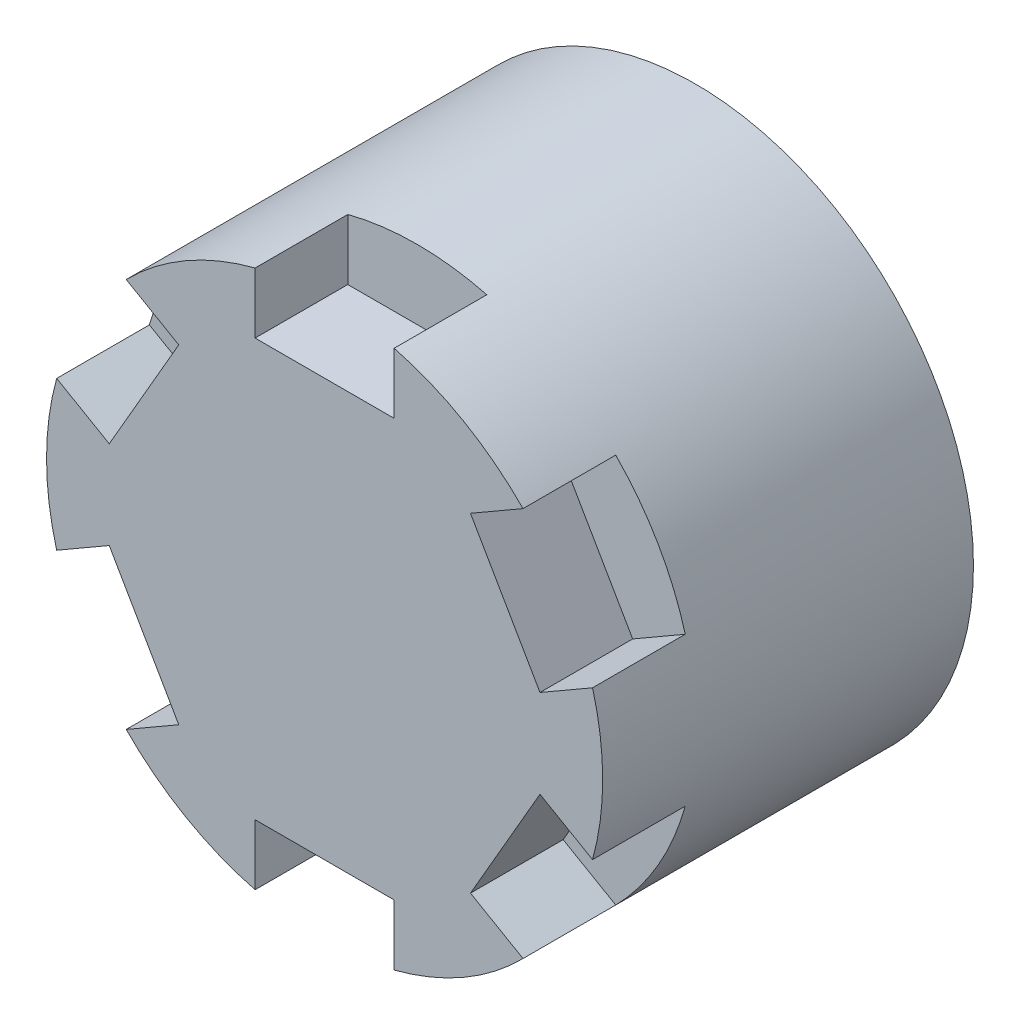
from build123d import *

# Parameters (mm, degrees)
SKETCH_2_R          = 60
EXTRUDE_1_DEPTH     = 80
SKETCH_1_R          = 37.5
CUT_EXTRUDE_1_DEPTH = 60
CUT_EXTRUDE_START   = -20
CUT_EXTRUDE_2_DEPTH = 20
SKETCH_4_W          = 20
SKETCH_4_H          = 11.668393693
CUT_EXTRUDE_3_DEPTH = 30


with BuildPart() as part:
    # 草图2 → 凸台-拉伸1 (new body)
    with BuildSketch(Plane.XY):
        Circle(SKETCH_2_R)
    extrude(amount=EXTRUDE_1_DEPTH)

    # 草图1 → 切除-拉伸1 (cut)
    with BuildSketch(Plane.XY):
        Circle(SKETCH_1_R)
    extrude(amount=CUT_EXTRUDE_1_DEPTH, mode=Mode.SUBTRACT)

    # 草图3 → 切除-拉伸2 (cut)
    with BuildSketch(Plane.XY.offset(80).offset(CUT_EXTRUDE_START)):
        with BuildLine():
            Line((57.811529494, 16.05699404), (46.47114317, 9.509618943))
            Line((46.47114317, 9.509618943), (31.47114317, 35.490381057))
            Line((31.47114317, 35.490381057), (42.811529494, 42.037756153))
            ThreePointArc((42.811529494, 42.037756153), (51.961524227, 30), (57.811529494, 16.05699404))
        make_face()
        with BuildLine():
            Line((-15, 58.094750193), (-15, 45))
            Line((-15, 45), (15, 45))
            Line((15, 45), (15, 58.094750193))
            ThreePointArc((15, 58.094750193), (0, 60), (-15, 58.094750193))
        make_face()
        with BuildLine():
            Line((42.811529494, -42.037756153), (31.47114317, -35.490381057))
            Line((31.47114317, -35.490381057), (46.47114317, -9.509618943))
            Line((46.47114317, -9.509618943), (57.811529494, -16.05699404))
            ThreePointArc((57.811529494, -16.05699404), (51.961524227, -30), (42.811529494, -42.037756153))
        make_face()
        with BuildLine():
            Line((-15, -58.094750193), (-15, -45))
            Line((-15, -45), (15, -45))
            Line((15, -45), (15, -58.094750193))
            ThreePointArc((15, -58.094750193), (0, -60), (-15, -58.094750193))
        make_face()
        with BuildLine():
            Line((-57.811529494, -16.05699404), (-46.47114317, -9.509618943))
            Line((-46.47114317, -9.509618943), (-31.47114317, -35.490381057))
            Line((-31.47114317, -35.490381057), (-42.811529494, -42.037756153))
            ThreePointArc((-42.811529494, -42.037756153), (-51.961524227, -30), (-57.811529494, -16.05699404))
        make_face()
        with BuildLine():
            Line((-42.811529494, 42.037756153), (-31.47114317, 35.490381057))
            Line((-31.47114317, 35.490381057), (-46.47114317, 9.509618943))
            Line((-46.47114317, 9.509618943), (-57.811529494, 16.05699404))
            ThreePointArc((-57.811529494, 16.05699404), (-51.961524227, 30), (-42.811529494, 42.037756153))
        make_face()
    extrude(amount=CUT_EXTRUDE_2_DEPTH, mode=Mode.SUBTRACT)

    # 草图4 → 切除-拉伸3 (cut)
    with BuildSketch(Plane(origin=(0, 0, 0), x_dir=(-1, 0, 0), z_dir=(0, 0, -1))):
        with Locations((0, 34.165803154)):
            Rectangle(SKETCH_4_W, SKETCH_4_H)
    extrude(amount=-CUT_EXTRUDE_3_DEPTH, mode=Mode.SUBTRACT)


solid = part.part
